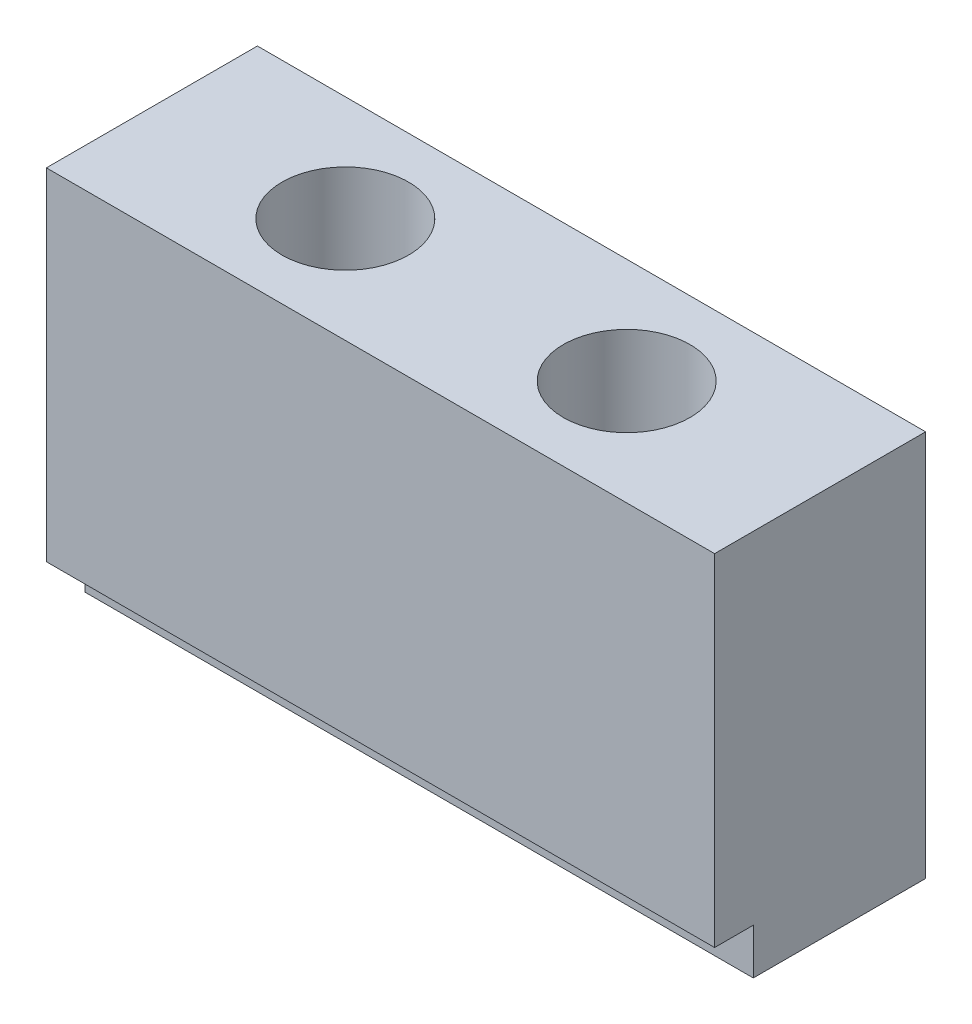
SolidWorks part; units mm, degrees
ref_plane "Front Plane" through (0, 0, 0) normal (0, 0, 1) x (1, 0, 0)
ref_plane "Top Plane" through (0, 0, 0) normal (0, 1, 0) x (1, 0, 0)
ref_plane "Right Plane" through (0, 0, 0) normal (1, 0, 0) x (0, 0, -1)
sketch "Sketch1" plane through (0, 0, 0) normal (0, 1, 0) x (1, 0, 0)
  line L1 (-47.5, -15) -> (47.5, -15)
  line L2 (-47.5, -15) -> (-47.5, 15)
  line L3 (-47.5, 15) -> (47.5, 15)
  line L4 (47.5, -15) -> (47.5, 15)
  line L5 (-47.5, -15) -> (47.5, 15) construction
  line L6 (-47.5, 15) -> (47.5, -15) construction
  point P0 (0, 0)
  dimension "D1" = 30
  dimension "D2" = 95
extrude "Boss-Extrude1" add sketch "Sketch1" along normal blind 55
sketch "Sketch2" plane through (0, 55, 0) normal (0, 1, 0) x (1, 0, 0)
  line L0 (47.5, -15) -> (47.5, 15) construction
  line L1 (-47.5, 15) -> (-47.5, -15) construction
  circle A0 centre (-20, 0) radius 5.5
  circle A1 centre (20, 0) radius 5.5
  dimension "D1" = 11
  dimension "D2" = 11
  dimension "D4" = 27.5
  dimension "D3" = 27.5
extrude "Cut-Extrude1" cut sketch "Sketch2" against normal through all
sketch "Sketch3" plane through (0, 55, 0) normal (0, 1, 0) x (1, 0, 0)
  circle A0 centre (-20, 0) radius 9
  circle A1 centre (20, 0) radius 9
  dimension "D1" = 18
  dimension "D2" = 18
extrude "Cut-Extrude2" cut sketch "Sketch3" against normal blind 20
sketch "Sketch4" plane through (-47.5, 0, 0) normal (-1, 0, 0) x (0, 0, 1)
  line L1 (15, 0) -> (9.5, 0)
  line L2 (15, 0) -> (15, 6.5)
  line L3 (15, 6.5) -> (9.5, 6.5)
  line L4 (9.5, 0) -> (9.5, 6.5)
  dimension "D1" = 6.5
  dimension "D2" = 5.5
extrude "Cut-Extrude3" cut sketch "Sketch4" against normal blind 172
